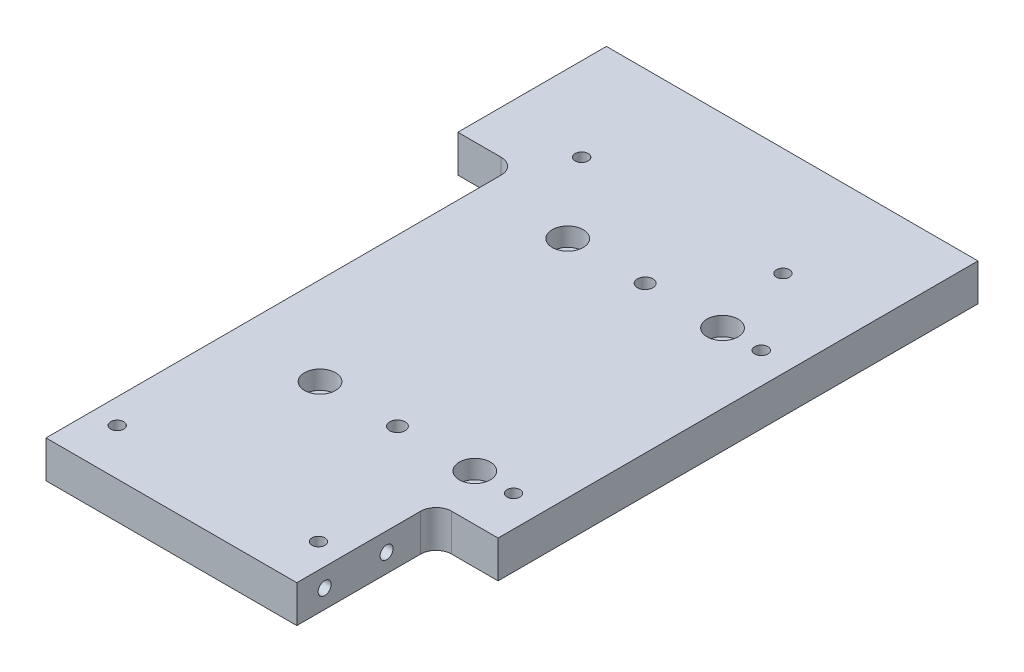
from build123d import *

# Parameters (mm, degrees)
SKETCH1_W                                         = 120
SKETCH1_H                                         = 200
EXTRUDE1_DEPTH                                    = 6
SKETCH3_W                                         = 19
SKETCH3_H                                         = 152
CUT_EXTRUDE1_DEPTH                                = 118.234807118
FILLET1_R                                         = 5
SKETCH4_W                                         = 20
SKETCH4_H                                         = 45
CUT_EXTRUDE2_DEPTH                                = 118.234807118
SKETCH6_R                                         = 2.5
CUT_EXTRUDE3_DEPTH                                = 118.234807118
M5_SOCKET_HEAD_CAP_SCREW_COUNTERBORE1_D           = 5.5
M5_SOCKET_HEAD_CAP_SCREW_COUNTERBORE1_CBORE_D     = 10
M5_SOCKET_HEAD_CAP_SCREW_COUNTERBORE1_CBORE_DEPTH = 6
M5_TAPPED_HOLE1_D                                 = 4.2
FILLET2_R                                         = 5
M5_TAPPED_HOLE2_D                                 = 4.2
M5_TAPPED_HOLE2_DEPTH                             = 12.4
M5_TAPPED_HOLE2_TIP                               = 1.2618073
M5_TAPPED_HOLE3_D                                 = 4.2


with BuildPart() as part:
    # Sketch1 → Extrude1 (new, symmetric)
    with BuildSketch(Plane(origin=(0, 0, 0), x_dir=(1, 0, 0), z_dir=(0, 1, 0))):
        Rectangle(SKETCH1_W, SKETCH1_H)
    extrude(amount=EXTRUDE1_DEPTH, both=True)

    # Sketch3 → Cut-Extrude1 (cut, through all)
    with BuildSketch(Plane(origin=(0, 6, 0), x_dir=(1, 0, 0), z_dir=(0, 1, 0))):
        with Locations((-50.5, -24)):
            Rectangle(SKETCH3_W, SKETCH3_H)
    extrude(amount=-CUT_EXTRUDE1_DEPTH, mode=Mode.SUBTRACT)

    # Fillet1
    fillet1_edges = [part.edges().sort_by_distance(p)[0] for p in [
        (-41, 0, -52),
    ]]
    fillet(fillet1_edges, radius=FILLET1_R)

    # Sketch4 → Cut-Extrude2 (cut, through all)
    with BuildSketch(Plane(origin=(0, 6, 0), x_dir=(1, 0, 0), z_dir=(0, 1, 0))):
        with Locations((50, -77.5)):
            Rectangle(SKETCH4_W, SKETCH4_H)
    extrude(amount=-CUT_EXTRUDE2_DEPTH, mode=Mode.SUBTRACT)

    # Sketch6 → Cut-Extrude3 (cut, through all)
    with BuildSketch(Plane(origin=(0, 6, 0), x_dir=(1, 0, 0), z_dir=(0, 1, 0))):
        with Locations(Location((12.5, 40, 0), (0, 0, 270))):
            Circle(SKETCH6_R)
        with Locations(Location((12.5, -40, 0), (0, 0, 270))):
            Circle(SKETCH6_R)
    extrude(amount=-CUT_EXTRUDE3_DEPTH, mode=Mode.SUBTRACT)

    # M5 Socket Head Cap Screw Counterbore1 (through all)
    with Locations(Plane(origin=(37.5, 6, -40), x_dir=(0, 0, 1), z_dir=(0, 1, 0))):
        with Locations((0, 0), (0, -50), (80, -50), (80, 0)):
            CounterBoreHole(M5_SOCKET_HEAD_CAP_SCREW_COUNTERBORE1_D / 2, M5_SOCKET_HEAD_CAP_SCREW_COUNTERBORE1_CBORE_D / 2, M5_SOCKET_HEAD_CAP_SCREW_COUNTERBORE1_CBORE_DEPTH)

    # M5 Tapped Hole1 (through all)
    with Locations(Plane(origin=(32, 6, 85), x_dir=(0, 0, 1), z_dir=(0, 1, 0))):
        with Locations((0, 0), (0, -65), (-150, 0), (-150, -65)):
            Hole(M5_TAPPED_HOLE1_D / 2)

    # Fillet2
    fillet2_edges = [part.edges().sort_by_distance(p)[0] for p in [
        (40, 0, 55),
    ]]
    fillet(fillet2_edges, radius=FILLET2_R)

    # M5 Tapped Hole2
    with Locations(Plane(origin=(40, 0, 91), x_dir=(0, 0, 1), z_dir=(1, 0, 0))):
        with Locations((0, 0), (-20, 0)):
            Hole(M5_TAPPED_HOLE2_D / 2, depth=M5_TAPPED_HOLE2_DEPTH)
            with Locations((0, 0, -(M5_TAPPED_HOLE2_DEPTH + M5_TAPPED_HOLE2_TIP / 2))):  # 118° drill point
                Cone(0, M5_TAPPED_HOLE2_D / 2, M5_TAPPED_HOLE2_TIP, mode=Mode.SUBTRACT)

    # M5 Tapped Hole3 (through all)
    with Locations(Plane(origin=(50, 6, -40), x_dir=(0, 0, 1), z_dir=(0, 1, 0))):
        with Locations((0, 0), (80, 0)):
            Hole(M5_TAPPED_HOLE3_D / 2)


solid = part.part
